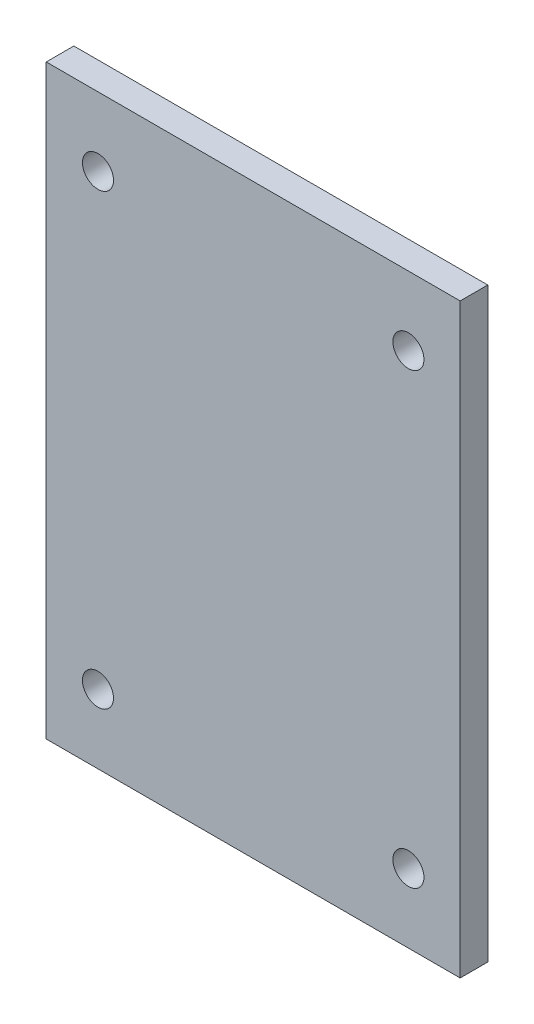
from build123d import *

# Parameters (mm, degrees)
SKETCH2_W           = 240
SKETCH2_H           = 340
SKETCH2_R           = 9
BOSS_EXTRUDE1_DEPTH = 16


with BuildPart() as part:
    # Sketch2 → Boss-Extrude1 (new body)
    with BuildSketch(Plane.XY):
        Rectangle(SKETCH2_W, SKETCH2_H)
        with Locations((-90, 130)):
            Circle(SKETCH2_R, mode=Mode.SUBTRACT)
        with Locations((90, 130)):
            Circle(SKETCH2_R, mode=Mode.SUBTRACT)
        with Locations((90, -130)):
            Circle(SKETCH2_R, mode=Mode.SUBTRACT)
        with Locations((-90, -130)):
            Circle(SKETCH2_R, mode=Mode.SUBTRACT)
    extrude(amount=BOSS_EXTRUDE1_DEPTH)


solid = part.part
